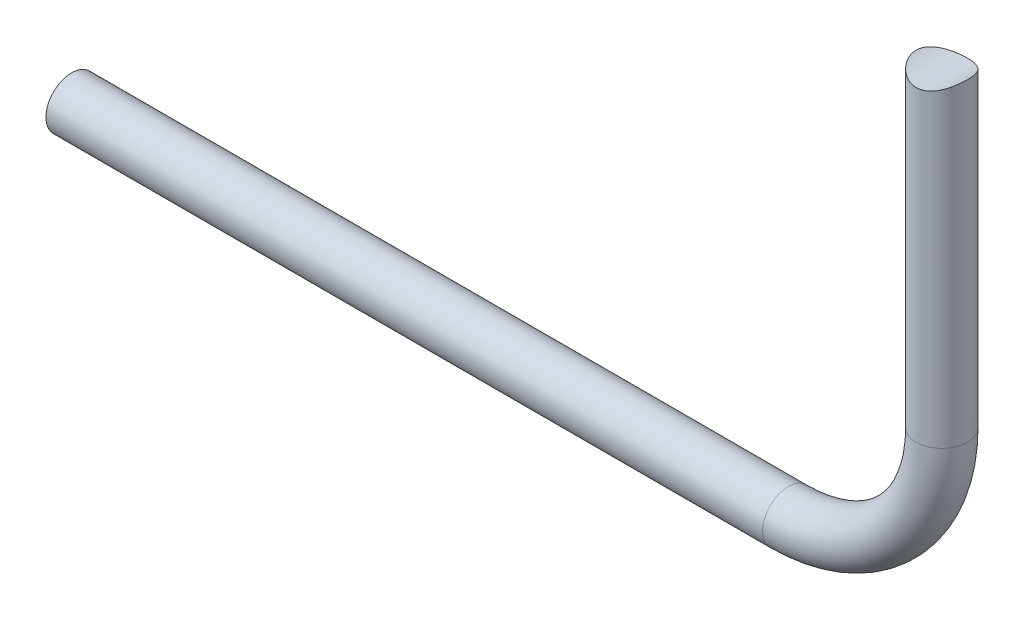
from build123d import *

# Parameters (mm, degrees)
SKETCH_2_R          = 5
SKETCH_3_R          = 10
CUT_EXTRUDE_1_DEPTH = 5


with BuildPart() as part:
    # 扫描1: sweep along a path in 草图1
    with BuildLine(Plane.XY) as sweep_1_path:
        Line((0, 0), (140, 0))
        ThreePointArc((140, 0), (161.213203436, 8.786796564), (170, 30))
        Line((170, 30), (170, 95))
    # 草图2 → 扫描1 (sweep)
    with BuildSketch(Plane(origin=(0, 0, 0), x_dir=(0, 0, -1), z_dir=(1, 0, 0))):
        Circle(SKETCH_2_R)
    sweep(path=sweep_1_path.line)

    # 草图3 → 切除-拉伸1 (cut, symmetric)
    with BuildSketch(Plane.XY):
        with Locations((170, 100)):
            Circle(SKETCH_3_R)
    extrude(amount=CUT_EXTRUDE_1_DEPTH, both=True, mode=Mode.SUBTRACT)


solid = part.part
